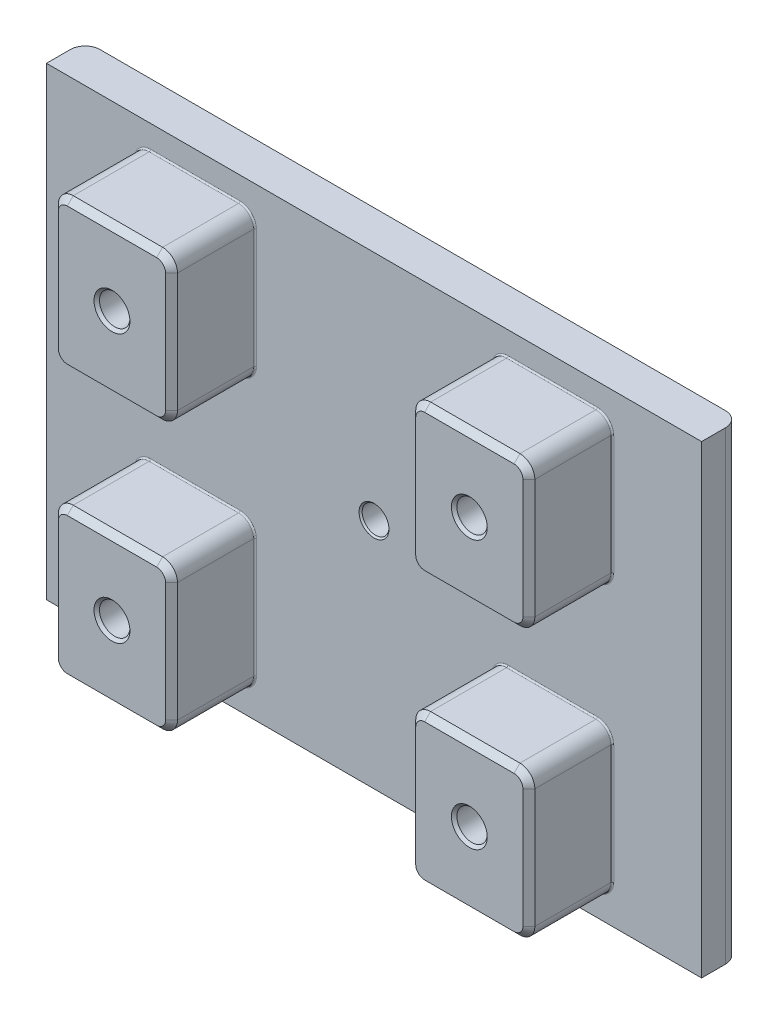
from build123d import *

# Parameters (mm, degrees)
SKETCH_1_W                    = 220
SKETCH_1_H                    = 156
EXTRUDE_1_DEPTH               = 13
SKETCH_2_W                    = 40
SKETCH_2_H                    = 50
EXTRUDE_2_DEPTH               = 28
FILLET_1_R                    = 5
HOLE_WIZARD_M12_1_D           = 10.2
HOLE_WIZARD_M12_1_DEPTH       = 30
HOLE_WIZARD_M12_1_CSINK_D     = 12.05
HOLE_WIZARD_M12_1_CSINK_ANGLE = 90
HOLE_WIZARD_M12_1_TIP         = 3.064389157
M10X1_0_1_D                   = 9
M10X1_0_1_DEPTH               = 25
M10X1_0_1_CSINK_D             = 10.05
M10X1_0_1_CSINK_ANGLE         = 90
M10X1_0_1_TIP                 = 2.703872786
FILLET_2_R                    = 5
CHAMFER_1_SIZE                = 2
CUT_EXTRUDE_1_DEPTH           = 1
CUT_EXTRUDE_2_DEPTH           = 1
FILLET_3_R                    = 0.5
FILLET_4_R                    = 1


with BuildPart() as part:
    # 草图1 → 凸台-拉伸1 (new body)
    with BuildSketch(Plane.XY):
        with Locations((110, -78)):
            Rectangle(SKETCH_1_W, SKETCH_1_H)
    extrude(amount=EXTRUDE_1_DEPTH)

    # 草图2 → 凸台-拉伸2 (add)
    with BuildSketch(Plane.XY.offset(13)):
        with Locations((50, -33)):
            Rectangle(SKETCH_2_W, SKETCH_2_H)
        with Locations((170, -33)):
            Rectangle(SKETCH_2_W, SKETCH_2_H)
        with Locations((170, -123)):
            Rectangle(SKETCH_2_W, SKETCH_2_H)
        with Locations((50, -123)):
            Rectangle(SKETCH_2_W, SKETCH_2_H)
    extrude(amount=EXTRUDE_2_DEPTH)

    # 圆角1
    fillet_1_edges = [part.edges().sort_by_distance(p)[0] for p in [
        (220, -78, 0),
        (0, -78, 0),
    ]]
    fillet(fillet_1_edges, radius=FILLET_1_R)

    # M12 螺纹孔1
    with Locations(Plane(origin=(50, -33, 41), x_dir=(1, 0, 0), z_dir=(0, 0, 1))):
        with Locations((0, 0), (120, 0), (120, -90), (0, -90)):
            CounterSinkHole(HOLE_WIZARD_M12_1_D / 2, HOLE_WIZARD_M12_1_CSINK_D / 2, depth=HOLE_WIZARD_M12_1_DEPTH, counter_sink_angle=HOLE_WIZARD_M12_1_CSINK_ANGLE)
            with Locations((0, 0, -(HOLE_WIZARD_M12_1_DEPTH + HOLE_WIZARD_M12_1_TIP / 2))):  # 118° drill point
                Cone(0, HOLE_WIZARD_M12_1_D / 2, HOLE_WIZARD_M12_1_TIP, mode=Mode.SUBTRACT)

    # M10x1.0 螺纹孔1
    with Locations(Plane(origin=(110, -78, 13), x_dir=(1, 0, 0), z_dir=(0, 0, 1))):
        with Locations((0, 0)):
            CounterSinkHole(M10X1_0_1_D / 2, M10X1_0_1_CSINK_D / 2, depth=M10X1_0_1_DEPTH, counter_sink_angle=M10X1_0_1_CSINK_ANGLE)
            with Locations((0, 0, -(M10X1_0_1_DEPTH + M10X1_0_1_TIP / 2))):  # 118° drill point
                Cone(0, M10X1_0_1_D / 2, M10X1_0_1_TIP, mode=Mode.SUBTRACT)

    # 圆角2
    fillet_2_edges = [part.edges().sort_by_distance(p)[0] for p in [
        (70, -58, 27),
        (70, -8, 27),
        (30, -8, 27),
        (30, -58, 27),
        (190, -8, 27),
        (150, -8, 27),
        (150, -58, 27),
        (190, -58, 27),
        (150, -148, 27),
        (190, -148, 27),
        (190, -98, 27),
        (150, -98, 27),
        (30, -98, 27),
        (30, -148, 27),
        (70, -148, 27),
        (70, -98, 27),
    ]]
    fillet(fillet_2_edges, radius=FILLET_2_R)

    # 倒角1
    chamfer_1_edges = [part.edges().sort_by_distance(p)[0] for p in [
        (50, -98, 41),
        (70, -123, 41),
        (30, -123, 41),
        (50, -148, 41),
        (68.535533906, -146.535533906, 41),
        (31.464466094, -146.535533906, 41),
        (31.464466094, -99.464466094, 41),
        (68.535533906, -99.464466094, 41),
        (170, -148, 41),
        (150, -123, 41),
        (190, -123, 41),
        (170, -98, 41),
        (151.464466094, -99.464466094, 41),
        (188.535533906, -99.464466094, 41),
        (188.535533906, -146.535533906, 41),
        (151.464466094, -146.535533906, 41),
        (150, -33, 41),
        (170, -8, 41),
        (170, -58, 41),
        (190, -33, 41),
        (151.464466094, -56.535533906, 41),
        (188.535533906, -56.535533906, 41),
        (188.535533906, -9.464466094, 41),
        (151.464466094, -9.464466094, 41),
        (70, -33, 41),
        (50, -58, 41),
        (50, -8, 41),
        (30, -33, 41),
        (31.464466094, -9.464466094, 41),
        (68.535533906, -9.464466094, 41),
        (31.464466094, -56.535533906, 41),
        (68.535533906, -56.535533906, 41),
    ]]
    chamfer(chamfer_1_edges, length=CHAMFER_1_SIZE)

    # 草图12 → 切除-拉伸1 (cut)
    with BuildSketch(Plane(origin=(0, 0, 0), x_dir=(-1, 0, 0), z_dir=(0, 0, -1))):
        with BuildLine():
            Line((-116, -128), (-116, -28))
            ThreePointArc((-116, -28), (-110, -22), (-104, -28))
            Line((-104, -28), (-104, -128))
            ThreePointArc((-104, -128), (-110, -134), (-116, -128))
        make_face()
    extrude(amount=-CUT_EXTRUDE_1_DEPTH, mode=Mode.SUBTRACT)

    # 草图13 → 切除-拉伸2 (cut)
    with BuildSketch(Plane(origin=(0, 0, 0), x_dir=(-1, 0, 0), z_dir=(0, 0, -1))):
        with BuildLine():
            Line((-185, -22), (-35, -22))
            ThreePointArc((-35, -22), (-29, -28), (-35, -34))
            Line((-35, -34), (-185, -34))
            ThreePointArc((-185, -34), (-191, -28), (-185, -22))
        make_face()
        with BuildLine():
            Line((-185, -134), (-35, -134))
            ThreePointArc((-35, -134), (-29, -128), (-35, -122))
            Line((-35, -122), (-185, -122))
            ThreePointArc((-185, -122), (-191, -128), (-185, -134))
        make_face()
    extrude(amount=-CUT_EXTRUDE_2_DEPTH, mode=Mode.SUBTRACT)

    # 圆角3
    fillet_3_edges = [part.edges().sort_by_distance(p)[0] for p in [
        (50, -98, 13),
        (70, -123, 13),
        (30, -123, 13),
        (50, -148, 13),
        (170, -148, 13),
        (150, -123, 13),
        (190, -123, 13),
        (170, -98, 13),
        (150, -33, 13),
        (170, -8, 13),
        (190, -33, 13),
        (170, -58, 13),
        (70, -33, 13),
        (50, -58, 13),
        (30, -33, 13),
        (50, -8, 13),
        (68.535533906, -99.464466094, 13),
        (31.464466094, -99.464466094, 13),
        (31.464466094, -146.535533906, 13),
        (68.535533906, -146.535533906, 13),
        (151.464466094, -146.535533906, 13),
        (188.535533906, -146.535533906, 13),
        (188.535533906, -99.464466094, 13),
        (151.464466094, -99.464466094, 13),
        (151.464466094, -9.464466094, 13),
        (188.535533906, -9.464466094, 13),
        (188.535533906, -56.535533906, 13),
        (151.464466094, -56.535533906, 13),
        (68.535533906, -56.535533906, 13),
        (31.464466094, -56.535533906, 13),
        (68.535533906, -9.464466094, 13),
        (31.464466094, -9.464466094, 13),
    ]]
    fillet(fillet_3_edges, radius=FILLET_3_R)

    # 圆角4
    fillet_4_edges = [part.edges().sort_by_distance(p)[0] for p in [
        (104, -122, 0.5),
        (104, -34, 0.5),
        (116, -34, 0.5),
        (116, -122, 0.5),
    ]]
    fillet(fillet_4_edges, radius=FILLET_4_R)


solid = part.part
